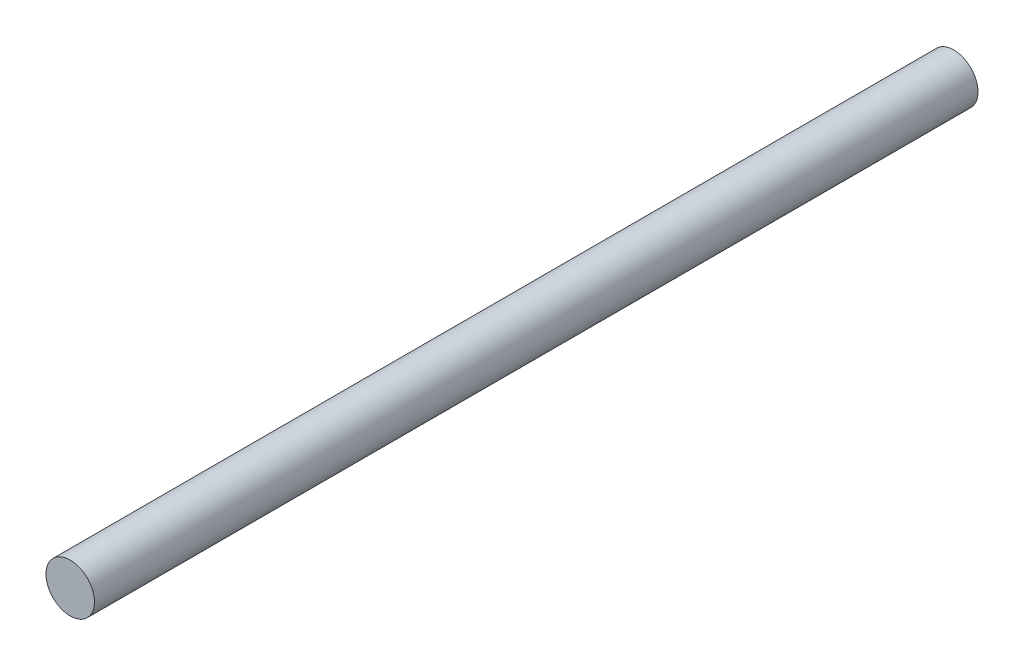
from build123d import *

# Parameters (mm, degrees)
SKETCH1_R           = 2.8
BOSS_EXTRUDE1_DEPTH = 102


with BuildPart() as part:
    # Sketch1 → Boss-Extrude1 (new body)
    with BuildSketch(Plane.XY):
        with Locations((-35, 4.7)):
            Circle(SKETCH1_R)
    extrude(amount=-BOSS_EXTRUDE1_DEPTH)


solid = part.part
